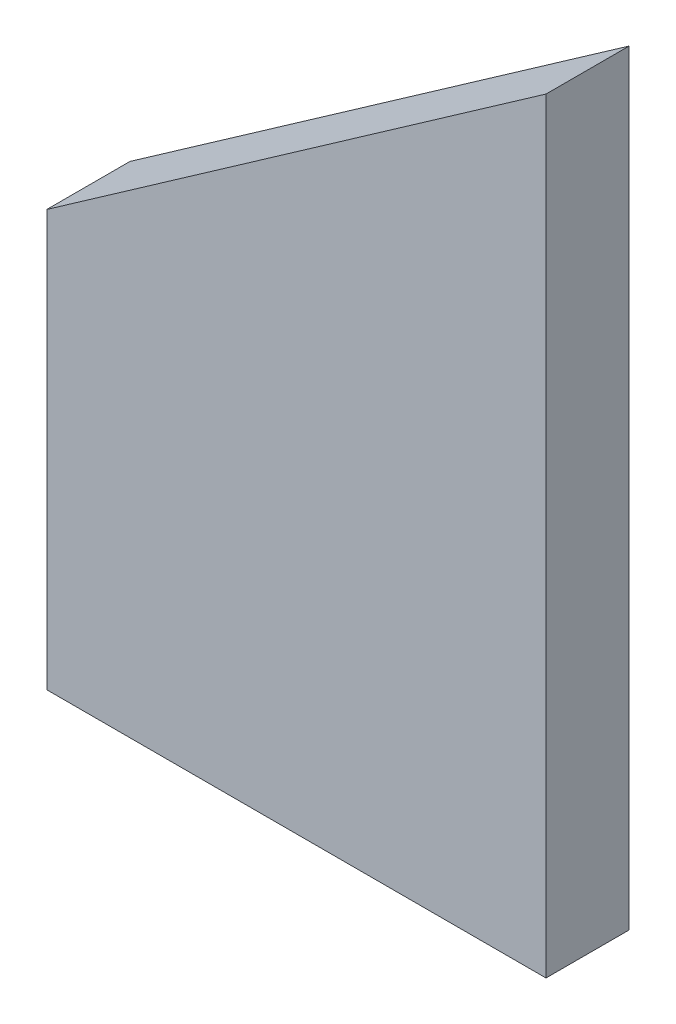
SolidWorks part; units mm, degrees
material "Q235-A "
ref_plane "前视基准面" through (0, 0, 0) normal (0, 0, 1) x (1, 0, 0)
ref_plane "上视基准面" through (0, 0, 0) normal (0, 1, 0) x (1, 0, 0)
ref_plane "右视基准面" through (0, 0, 0) normal (1, 0, 0) x (0, 0, -1)
sketch "草图1" plane through (0, 0, 0) normal (0, 0, 1) x (1, 0, 0)
  line L0 (-97.1613, 188.969) -> (-133.7109, 163.3767) construction
  line L1 (-102, 95.3473) -> (-102, 185.5809) construction
  line L2 (-102, 41.1328) -> (-102, 121.3353) construction
  line L3 (-97.1613, 188.969) -> (-52.6203, 220.157) construction
  line L5 (-102, 125.5809) -> (-102, 185.5809)
  line L6 (-102, 185.5809) -> (-30, 235.9958)
  line L7 (-30, 235.9958) -> (-30, 125.5809)
  line L8 (-30, 41.1328) -> (-30, 121.3353) construction
  line L9 (-30, 125.5809) -> (-102, 125.5809)
  dimension "D1" = 60
extrude "凸台-拉伸1" add sketch "草图1" along normal blind 12 from offset 260 offset against normal yes
